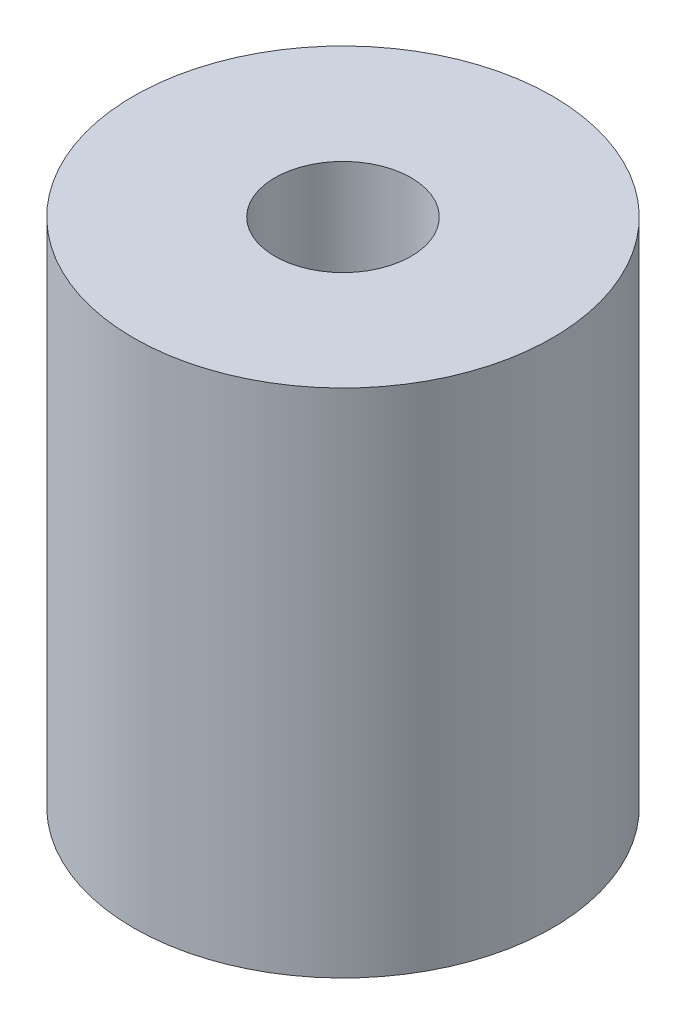
SolidWorks part; units mm, degrees
ref_plane "前视基准面" through (0, 0, 0) normal (0, 0, 1) x (1, 0, 0)
ref_plane "上视基准面" through (0, 0, 0) normal (0, 1, 0) x (1, 0, 0)
ref_plane "右视基准面" through (0, 0, 0) normal (1, 0, 0) x (0, 0, -1)
sketch "草图1" plane through (0, 0, 0) normal (0, 0, 1) x (1, 0, 0)
  line L0 (0, 0) -> (0, 6283.3549) construction
  line L1 (4, 25.7473) -> (12.3, 25.7473)
  line L2 (12.3, 25.7473) -> (12.3, -4.2527)
  line L3 (12.3, -4.2527) -> (4, -4.2527)
  line L4 (4, -4.2527) -> (4, 25.7473)
  dimension "D1" = 4
  dimension "D2" = 30
  dimension "D3" = 8.3
revolve "旋转1" add sketch "草图1" angle 360 about L0
